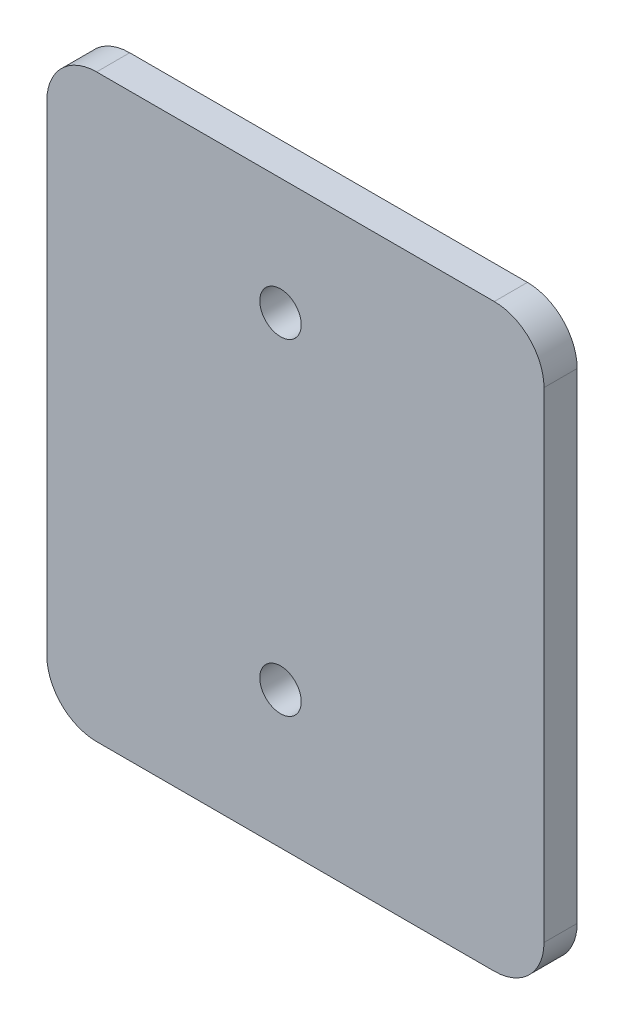
from build123d import *

# Parameters (mm, degrees)
SKETCH1_W           = 30
SKETCH1_H           = 35
BOSS_EXTRUDE1_DEPTH = 2
FILLET1_R           = 3
M3_TAPPED_HOLE1_D   = 2.5


with BuildPart() as part:
    # Sketch1 → Boss-Extrude1 (new body)
    with BuildSketch(Plane.XY):
        with Locations((-72.289490021, -50.654966575)):
            Rectangle(SKETCH1_W, SKETCH1_H)
    extrude(amount=BOSS_EXTRUDE1_DEPTH)

    # Fillet1
    fillet1_edges = [part.edges().sort_by_distance(p)[0] for p in [
        (-87.289490021, -33.154966575, 1),
        (-57.289490021, -33.154966575, 1),
        (-57.289490021, -68.154966575, 1),
        (-87.289490021, -68.154966575, 1),
    ]]
    fillet(fillet1_edges, radius=FILLET1_R)

    # M3 Tapped Hole1 (through all)
    with Locations(Plane.XY.offset(2)):
        with Locations((-73.189490021, -59.894365688), (-73.189490021, -40.194365688)):
            Hole(M3_TAPPED_HOLE1_D / 2)


solid = part.part
